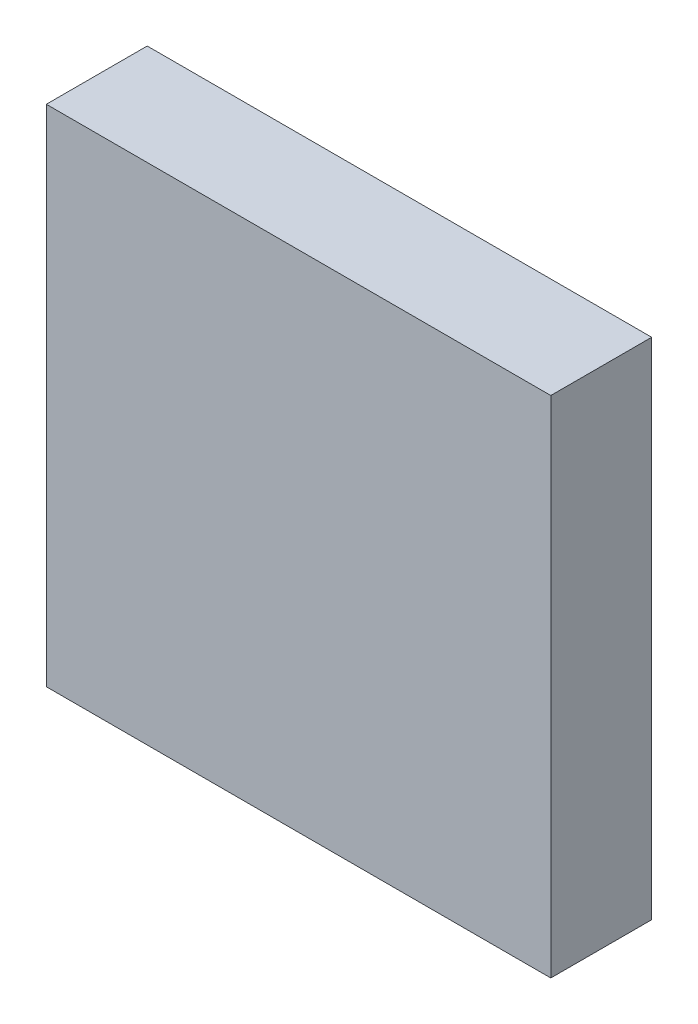
from build123d import *

# Parameters (mm, degrees)
SKETCH1_W           = 80
SKETCH1_H           = 80
BOSS_EXTRUDE1_DEPTH = 16


with BuildPart() as part:
    # Sketch1 → Boss-Extrude1 (new body)
    with BuildSketch(Plane.XY):
        Rectangle(SKETCH1_W, SKETCH1_H)
    extrude(amount=BOSS_EXTRUDE1_DEPTH)


solid = part.part
